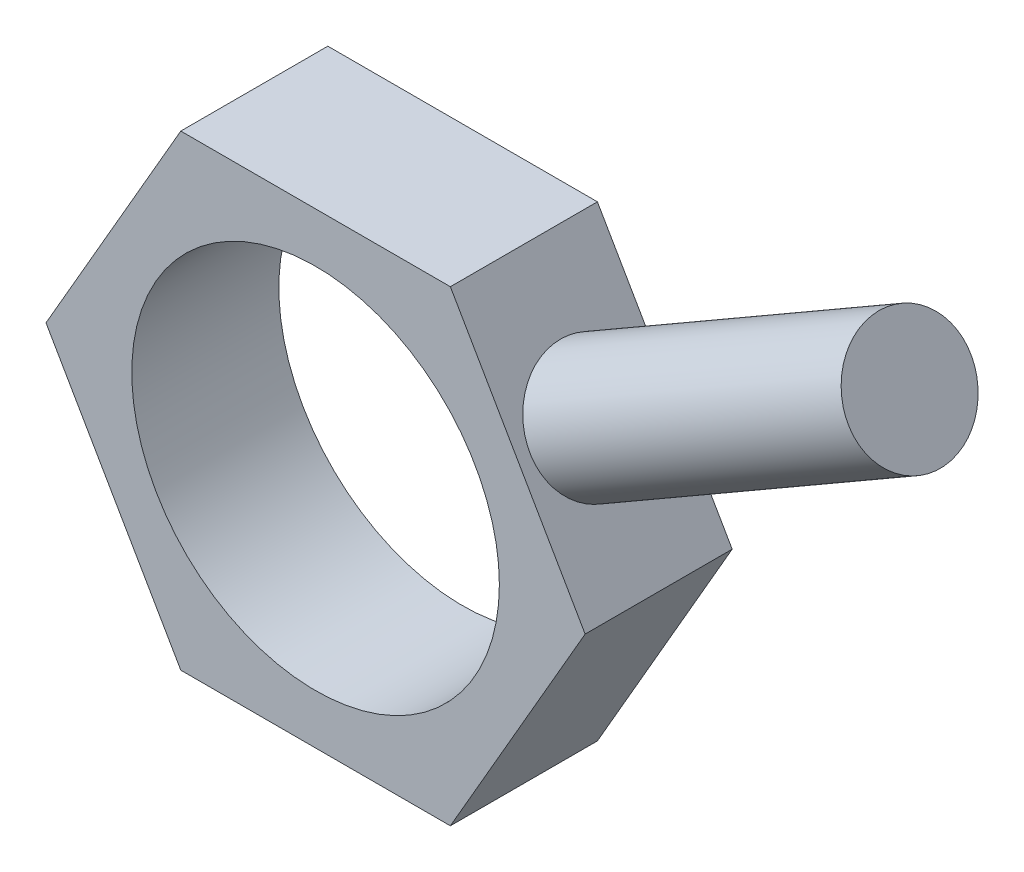
SolidWorks part; units mm, degrees
ref_plane "Front Plane" through (0, 0, 0) normal (0, 0, 1) x (1, 0, 0)
ref_plane "Top Plane" through (0, 0, 0) normal (0, 1, 0) x (1, 0, 0)
ref_plane "Right Plane" through (0, 0, 0) normal (1, 0, 0) x (0, 0, -1)
sketch "Sketch1" plane through (0, 0, 0) normal (0, 0, 1) x (1, 0, 0)
  line L1 (-5.5, 9.5263) -> (-11, 0)
  line L2 (-11, 0) -> (-5.5, -9.5263)
  line L3 (-5.5, -9.5263) -> (5.5, -9.5263)
  line L4 (5.5, -9.5263) -> (11, 0)
  line L5 (11, 0) -> (5.5, 9.5263)
  line L6 (5.5, 9.5263) -> (-5.5, 9.5263)
  circle A0 centre (0, 0) radius 7.5
  circle A1 centre (0, 0) radius 9.5263 construction
  dimension "D1" = 15
  dimension "D2" = 22
extrude "Boss-Extrude1" add sketch "Sketch1" along normal blind 6
sketch "Sketch2" plane through (8.25, 4.7631, 0) normal (0.866, 0.5, 0) x (0, 0, -1)
  line L0 (-6, 5.5) -> (0, 5.5) construction
  circle A0 centre (-3, 0) radius 2.5
  point P4 (-3, 5.5)
  dimension "D1" = 5
extrude "Boss-Extrude2" add sketch "Sketch2" along normal blind 15
